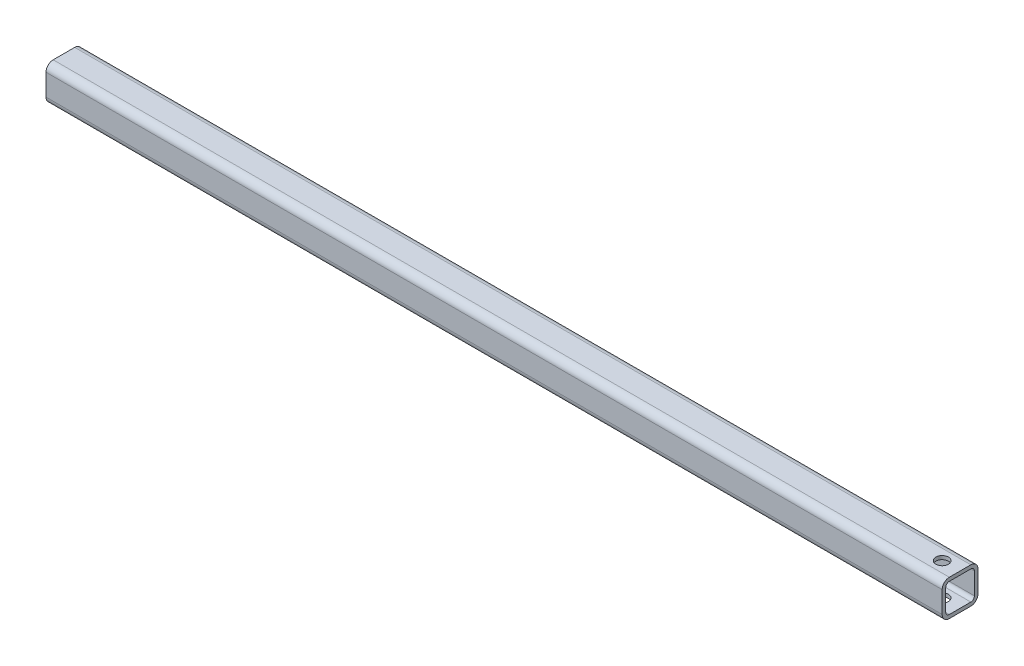
from build123d import *

# Parameters (mm, degrees)
GB_6728_1986_040_X_40_X_4_1_DEPTH = 1000
HOLE_WIZARD_M16_1_D               = 14


with BuildPart() as part:
    # Sketch12 → Gb／6728-1986方形空心型钢 040 X 40 X 4(1) (new body)
    with BuildSketch(Plane.ZY):
        with BuildLine():
            Line((-12, -20), (12, -20))
            ThreePointArc((12, -20), (17.656854249, -17.656854249), (20, -12))
            Line((20, -12), (20, 12))
            ThreePointArc((20, 12), (17.656854249, 17.656854249), (12, 20))
            Line((12, 20), (-12, 20))
            ThreePointArc((-12, 20), (-17.656854249, 17.656854249), (-20, 12))
            Line((-20, 12), (-20, -12))
            ThreePointArc((-20, -12), (-17.656854249, -17.656854249), (-12, -20))
        make_face()
        with BuildLine():
            Line((-12, -16), (12, -16))
            ThreePointArc((12, -16), (14.828427125, -14.828427125), (16, -12))
            Line((16, -12), (16, 12))
            ThreePointArc((16, 12), (14.828427125, 14.828427125), (12, 16))
            Line((12, 16), (-12, 16))
            ThreePointArc((-12, 16), (-14.828427125, 14.828427125), (-16, 12))
            Line((-16, 12), (-16, -12))
            ThreePointArc((-16, -12), (-14.828427125, -14.828427125), (-12, -16))
        make_face(mode=Mode.SUBTRACT)
    extrude(amount=GB_6728_1986_040_X_40_X_4_1_DEPTH)

    # M16 螺纹孔1 (through all)
    with Locations(Plane(origin=(0, 20, 0), x_dir=(1, 0, 0), z_dir=(0, 1, 0))):
        with Locations((-20, 0)):
            Hole(HOLE_WIZARD_M16_1_D / 2)


solid = part.part
